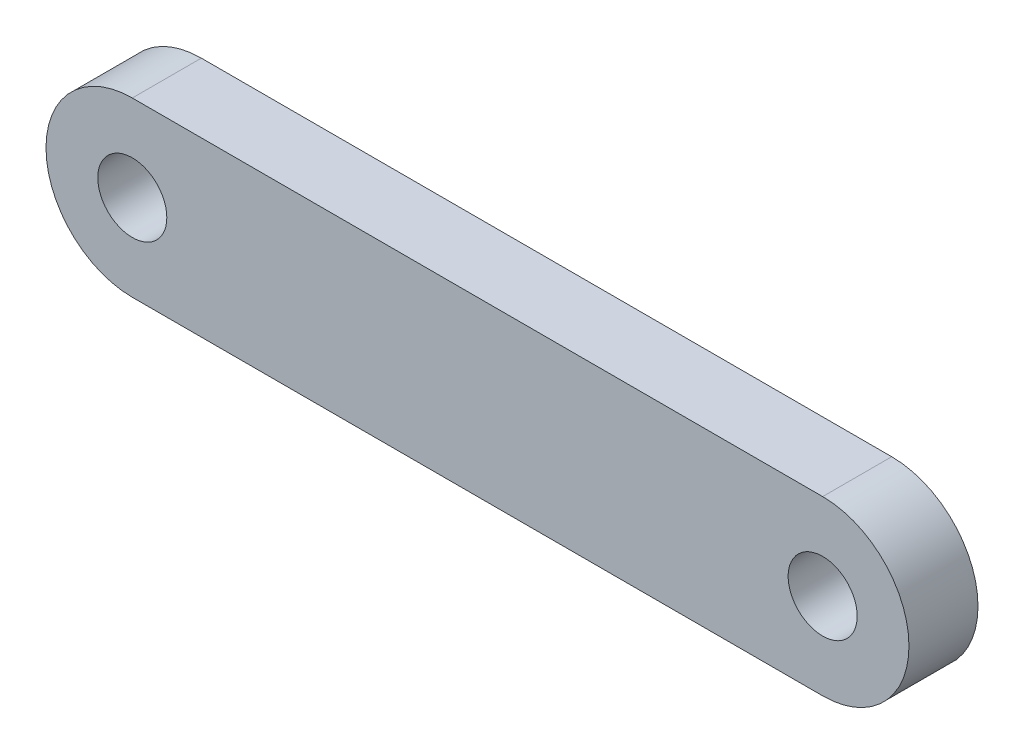
SolidWorks part; units mm, degrees
ref_plane "Front Plane" through (0, 0, 0) normal (0, 0, 1) x (1, 0, 0)
ref_plane "Top Plane" through (0, 0, 0) normal (0, 1, 0) x (1, 0, 0)
ref_plane "Right Plane" through (0, 0, 0) normal (1, 0, 0) x (0, 0, -1)
other "Configuration Table"
sketch "Sketch1" plane through (0, 0, 0) normal (0, 0, 1) x (1, 0, 0)
  line L0 (0, 0) -> (60, 0) construction
  line L1 (0, 7.5) -> (60, 7.5)
  line L2 (0, -7.5) -> (60, -7.5)
  arc A0 (0, 7.5) -> (0, -7.5) centre (0, 0) ccw
  arc A1 (60, -7.5) -> (60, 7.5) centre (60, 0) ccw
  circle A2 centre (0, 0) radius 3
  circle A3 centre (60, 0) radius 3
  point P3 (30, 0)
  dimension "D3" = 6
  dimension "D4" = 6
  dimension "D1" = 60
  dimension "D2" = 15
extrude "Boss-Extrude1" add sketch "Sketch1" along normal blind 6
